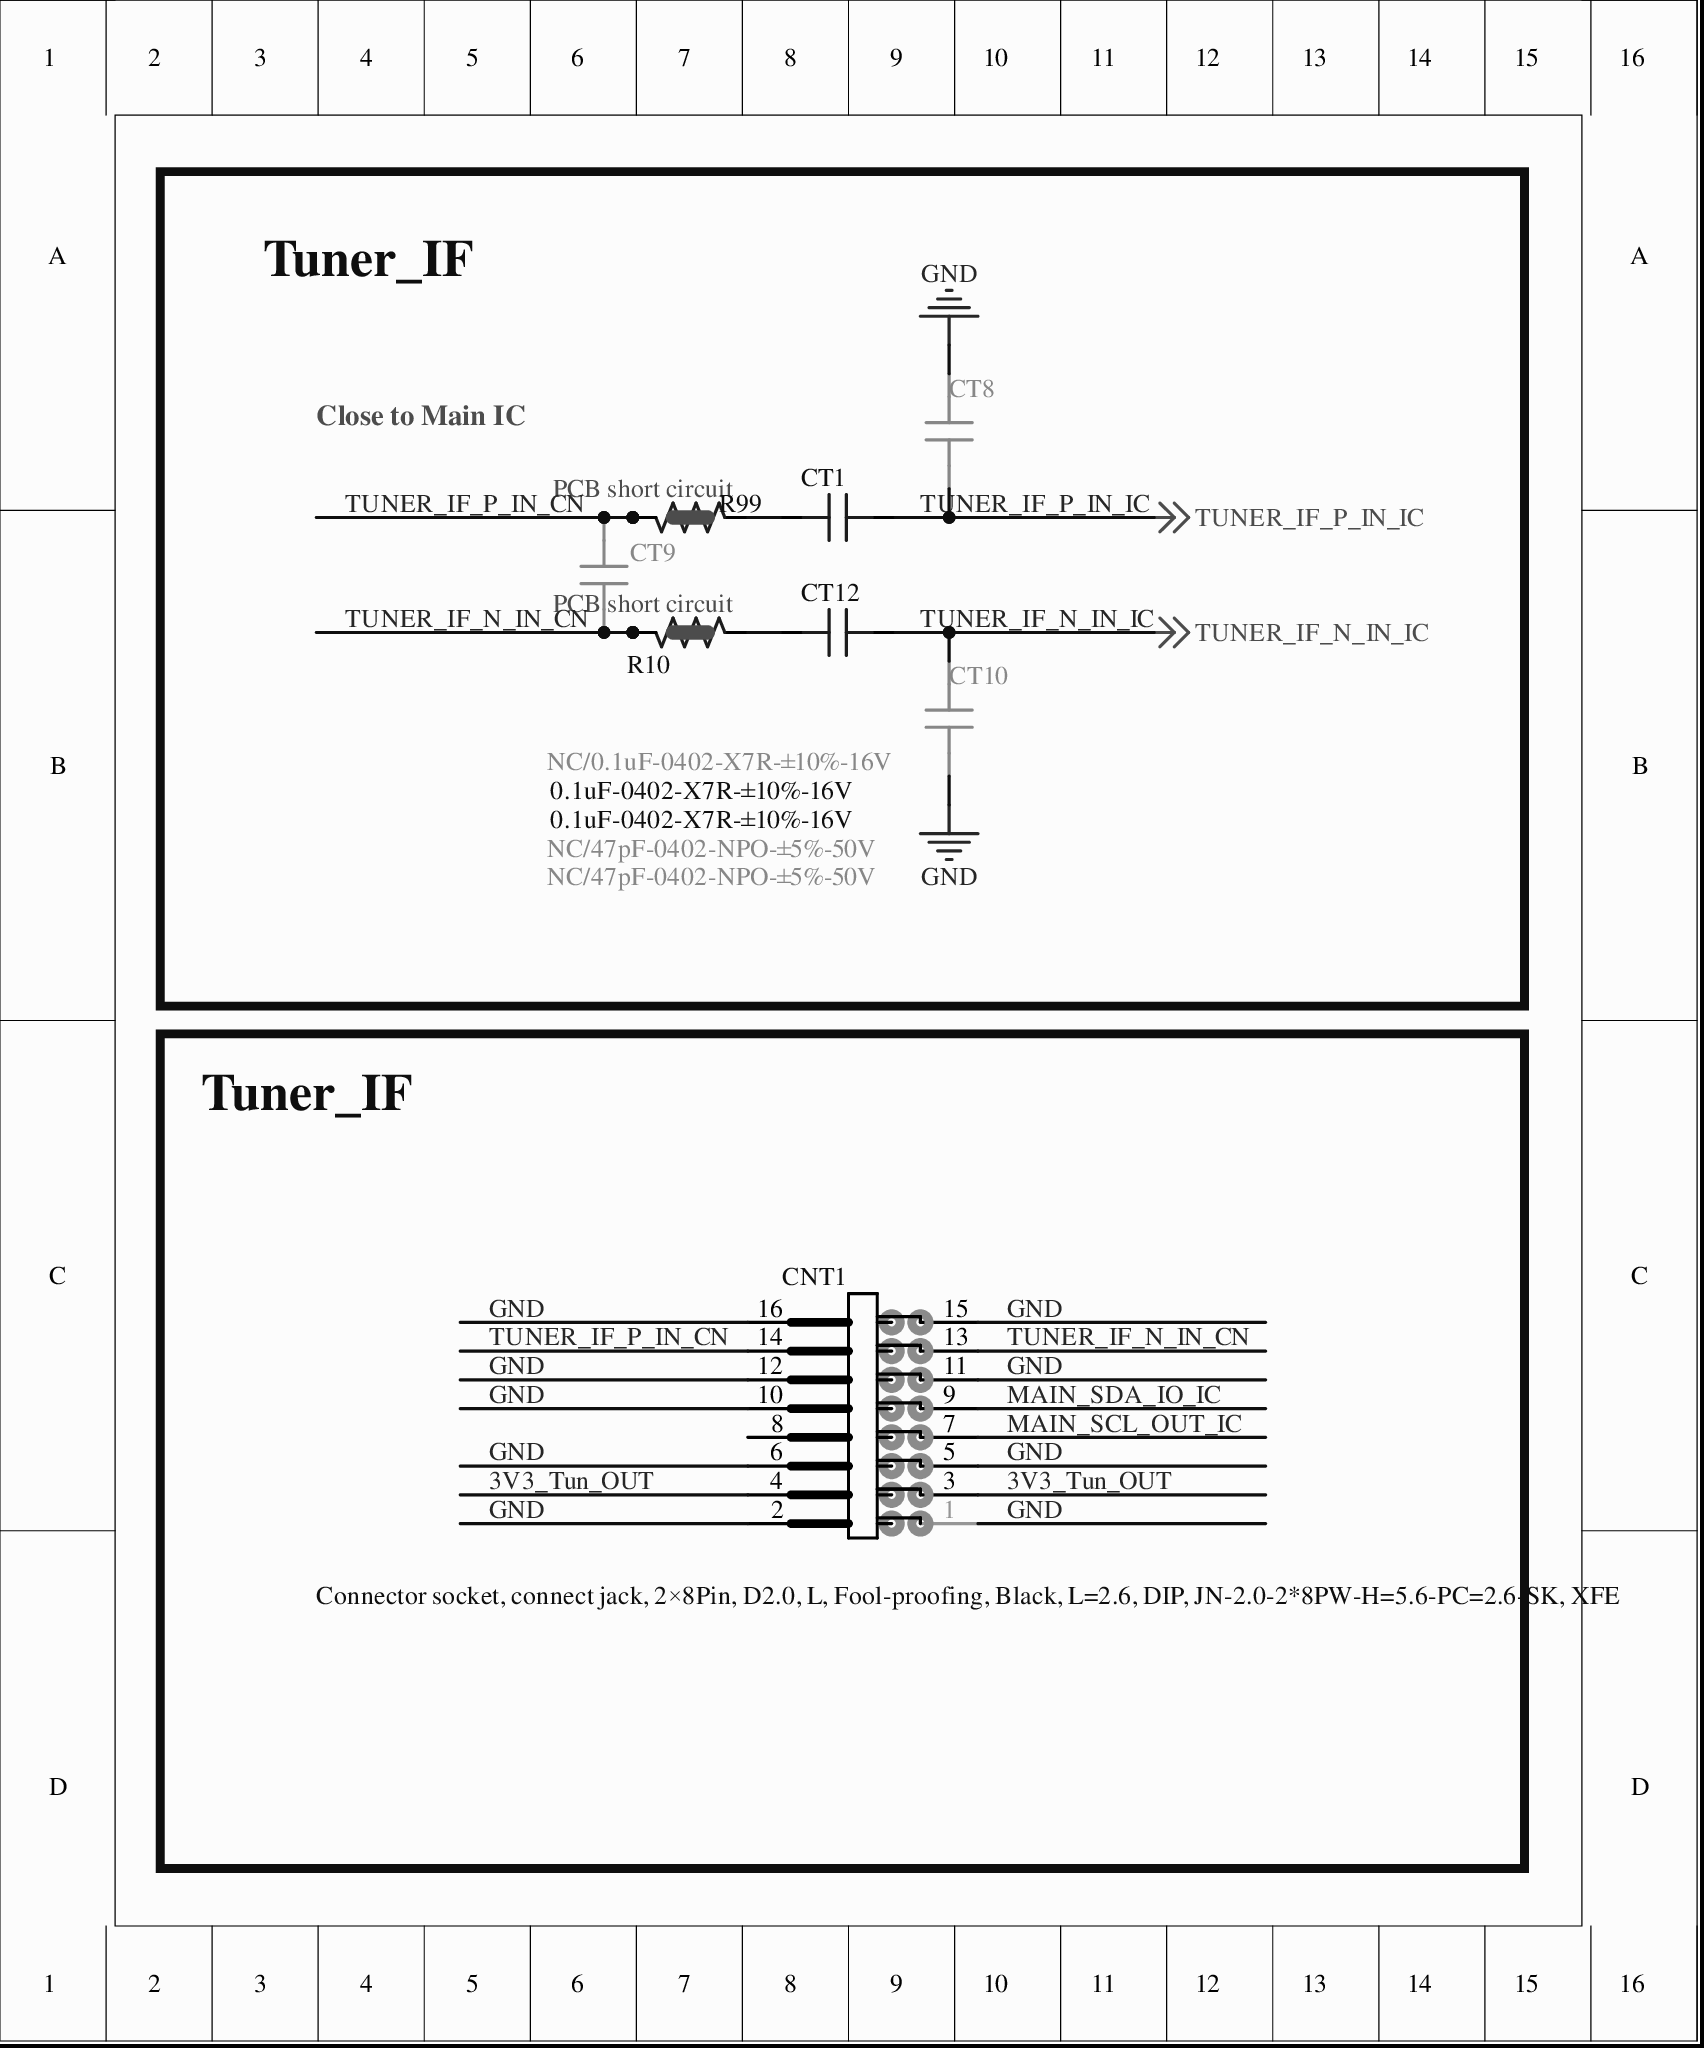
[diagram p0: MISC105950-42.SchDoc]
# Altium project MISC105950-48.PrjPCB (part 8 of 8)

## Sheet MISC105950-42.SchDoc
size 149 x 180 mm

### Parts
CNT1  Connector socket, connect jack, 2×8Pin, D2.0, L, Fool-proofing, Black, L=2.6, DIP, JN-2.0-2*8PW-H=5.6-PC=2.6-SK, XFE  [SIP2*8H/2.0DM-1]
CT1  0.1uF-0402-X7R-±10%-16V  [C0402]
CT8  NC/47pF-0402-NPO-±5%-50V  [C0402]
CT9  NC/0.1uF-0402-X7R-±10%-16V  [C0402]
CT10  NC/47pF-0402-NPO-±5%-50V  [C0402]
CT12  0.1uF-0402-X7R-±10%-16V  [C0402]
R10  NC/0ohm-0402-PCB  [R0402SC]  (value not drawn)
R99  NC/0ohm-0402-PCB  [R0402SC]  (value not drawn)

### Blocks framed on the sheet
Tuner_IF: CT1 CT8-CT10 CT12 R10 R99
Tuner_IF: CNT1

### Nets
3V3_Tun_OUT: CNT1.3 CNT1.4
GND: CNT1.1 CNT1.2 CNT1.5 CNT1.6 CNT1.10 CNT1.11 CNT1.12 CNT1.15 CNT1.16 CT8.1 CT10.2
MAIN_SCL_OUT_IC: CNT1.7
MAIN_SDA_IO_IC: CNT1.9
TUNER_IF_N_IN_CN: CNT1.13 CT9.1 R10.2 R10.3
TUNER_IF_N_IN_IC: CT10.1 CT12.1 ; off-sheet TUNER_IF_N_IN_IC
TUNER_IF_P_IN_CN: CNT1.14 CT9.2 R99.2 R99.3
TUNER_IF_P_IN_IC: CT1.1 CT8.2 ; off-sheet TUNER_IF_P_IN_IC
NetCT1_2: CT1.2 R99.1
NetCT12_2: CT12.2 R10.1

Not connected (* = marked no-connect by the designer): CNT1 8*

### Notes on the sheet
- Close to Main IC

### Library data of the parts
CNT1 = 连接插座-公座,male connect jack,2×8Pin,D2.0,L,Fool-proofing,Black,L=3.0mm,DIP,LK-DLMI
CT1 CT9 CT12 = 004.003.0000403-D: Ceramic capacitor, CAP MC, 16V, 0.1uF, ±20%, X5R, 0402, SMD, TP-D
CT8 CT10 = 004.003.0000556-D: Ceramic capacitor, CAP MC, 50V, 47pF, ±5%, NPO, 0402, SMD, TP-D
R10 R99 = 0ohm-0402-PCB-D

## Sheet MISC105950-43.SchDoc
size 416 x 279 mm
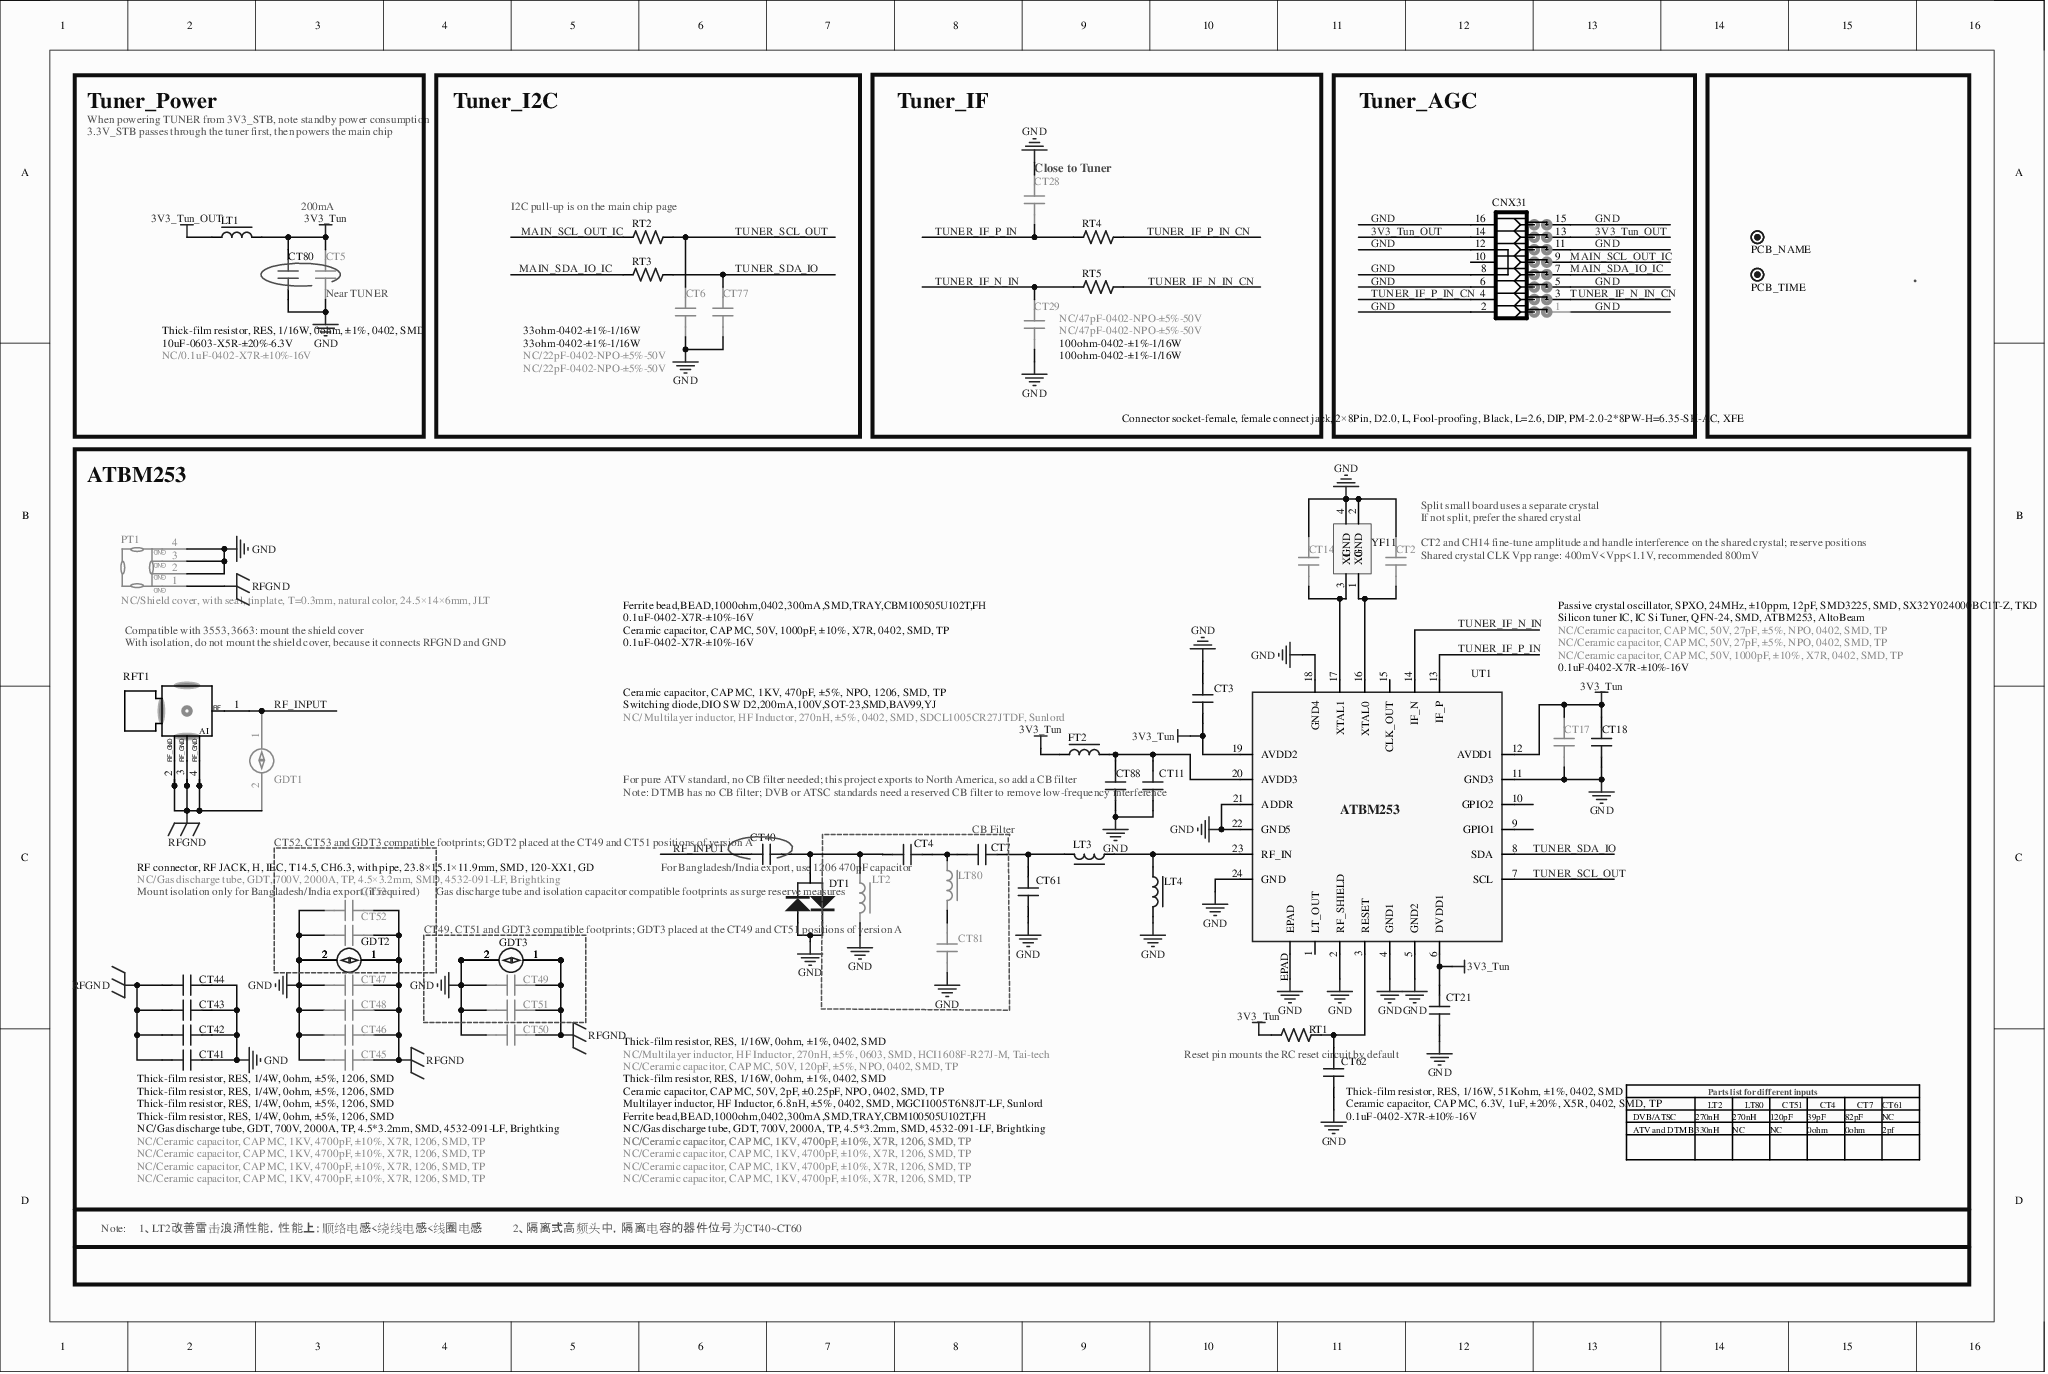
[diagram p1: MISC105950-43.SchDoc]

### Parts
CNX31  Connector socket-female, female connect jack, 2×8Pin, D2.0, L, Fool-proofing, Black, L=2.6, DIP, PM-2.0-2*8PW-H=6.35-SK-AC, XFE  [SIP2*8H/2.0DF-1]
CT2  NC/Ceramic capacitor, CAP MC, 50V, 27pF, ±5%, NPO, 0402, SMD, TP  [C0402]
CT3  0.1uF-0402-X7R-±10%-16V  [C0402]
CT4  Thick-film resistor, RES, 1/16W, 0ohm, ±1%, 0402, SMD  [C0402]
CT5  NC/0.1uF-0402-X7R-±10%-16V  [C0402]
CT6  NC/22pF-0402-NPO-±5%-50V  [C0402]
CT7  Thick-film resistor, RES, 1/16W, 0ohm, ±1%, 0402, SMD  [C0402]
CT11  Ceramic capacitor, CAP MC, 50V, 1000pF, ±10%, X7R, 0402, SMD, TP  [C0402]
CT14  NC/Ceramic capacitor, CAP MC, 50V, 27pF, ±5%, NPO, 0402, SMD, TP  [C0402]
CT17  NC/Ceramic capacitor, CAP MC, 50V, 1000pF, ±10%, X7R, 0402, SMD, TP  [C0402]
CT18  0.1uF-0402-X7R-±10%-16V  [C0402]
CT21  0.1uF-0402-X7R-±10%-16V  [C0402]
CT28  NC/47pF-0402-NPO-±5%-50V  [C0402]
CT29  NC/47pF-0402-NPO-±5%-50V  [C0402]
CT40  Ceramic capacitor, CAP MC, 1KV, 470pF, ±5%, NPO, 1206, SMD, TP  [C1206]
CT41  Thick-film resistor, RES, 1/4W, 0ohm, ±5%, 1206, SMD  [C1206]
CT42  Thick-film resistor, RES, 1/4W, 0ohm, ±5%, 1206, SMD  [C1206]
CT43  Thick-film resistor, RES, 1/4W, 0ohm, ±5%, 1206, SMD  [C1206]
CT44  Thick-film resistor, RES, 1/4W, 0ohm, ±5%, 1206, SMD  [C1206]
CT45  NC/Ceramic capacitor, CAP MC, 1KV, 4700pF, ±10%, X7R, 1206, SMD, TP  [C1206]
CT46  NC/Ceramic capacitor, CAP MC, 1KV, 4700pF, ±10%, X7R, 1206, SMD, TP  [C1206]
CT47  NC/Ceramic capacitor, CAP MC, 1KV, 4700pF, ±10%, X7R, 1206, SMD, TP  [C1206]
CT48  NC/Ceramic capacitor, CAP MC, 1KV, 4700pF, ±10%, X7R, 1206, SMD, TP  [C1206]
CT49  NC/Ceramic capacitor, CAP MC, 1KV, 4700pF, ±10%, X7R, 1206, SMD, TP  [C1206]
CT50  NC/Ceramic capacitor, CAP MC, 1KV, 4700pF, ±10%, X7R, 1206, SMD, TP  [C1206]
CT51  NC/Ceramic capacitor, CAP MC, 1KV, 4700pF, ±10%, X7R, 1206, SMD, TP  [C1206]
CT52  NC/Ceramic capacitor, CAP MC, 1KV, 4700pF, ±10%, X7R, 1206, SMD, TP  [C1206]
CT53  NC/Ceramic capacitor, CAP MC, 1KV, 4700pF, ±10%, X7R, 1206, SMD, TP  [C1206]
CT61  Ceramic capacitor, CAP MC, 50V, 2pF, ±0.25pF, NPO, 0402, SMD, TP  [C0402]
CT62  Ceramic capacitor, CAP MC, 6.3V, 1uF, ±20%, X5R, 0402, SMD, TP  [C0402]
CT77  NC/22pF-0402-NPO-±5%-50V  [C0402]
CT80  10uF-0603-X5R-±20%-6.3V  [C0603]
CT81  NC/Ceramic capacitor, CAP MC, 50V, 120pF, ±5%, NPO, 0402, SMD, TP  [C0402]
CT88  0.1uF-0402-X7R-±10%-16V  [C0402]
DT1  Switching diode,DIO SW D2,200mA,100V,SOT-23,SMD,BAV99,YJ  [SO-23]
FT2  Ferrite bead,BEAD,1000ohm,0402,300mA,SMD,TRAY,CBM100505U102T,FH  [L0402]
GDT1  NC/Gas discharge tube, GDT, 700V, 2000A, TP, 4.5×3.2mm, SMD, 4532-091-LF, Brightking  [SMD4532-1]
GDT2  NC/Gas discharge tube, GDT, 700V, 2000A, TP, 4.5*3.2mm, SMD, 4532-091-LF, Brightking  [SMD4532-1-C1206]
GDT3  NC/Gas discharge tube, GDT, 700V, 2000A, TP, 4.5*3.2mm, SMD, 4532-091-LF, Brightking  [SMD4532-1-C1206]
LT1  Thick-film resistor, RES, 1/16W, 0ohm, ±1%, 0402, SMD  [L0402]
LT2  NC/ Multilayer inductor, HF Inductor, 270nH, ±5%, 0402, SMD, SDCL1005CR27JTDF, Sunlord  [L0402]
LT3  Multilayer inductor, HF Inductor, 6.8nH, ±5%, 0402, SMD, MGCI1005T6N8JT-LF, Sunlord  [L0402]
LT4  Ferrite bead,BEAD,1000ohm,0402,300mA,SMD,TRAY,CBM100505U102T,FH  [L0402]
LT80  NC/Multilayer inductor, HF Inductor, 270nH, ±5%, 0603, SMD, HCI1608F-R27J-M, Tai-tech  [L0603]
PT1  NC/Shield cover, with seal, tinplate, T=0.3mm, natural color, 24.5×14×6mm, JLT  [SHIELD(24.5*14*6)-TEMP-NG]
RFT1  RF connector, RF JACK, H, IEC, T14.5, CH6.3, with pipe, 23.8×15.1×11.9mm, SMD, 120-XX1, GD  [T-12.8×10×9.3-IEC14.5-6.3]
RT1  Thick-film resistor, RES, 1/16W, 51Kohm, ±1%, 0402, SMD  [R0402]
RT2  33ohm-0402-±1%-1/16W  [R0402]
RT3  33ohm-0402-±1%-1/16W  [R0402]
RT4  100ohm-0402-±1%-1/16W  [R0402]
RT5  100ohm-0402-±1%-1/16W  [R0402]
UT1  Silicon tuner IC, IC Si Tuner, QFN-24, SMD, ATBM253, AltoBeam  [QFN24/0.4-1]
XX.XXXX  PCB_NAME  [PCB_NAME]
XXXXXX.  PCB_TIME  [PCB_TIME]
YF11  Passive crystal oscillator, SPXO, 24MHz, ±10ppm, 12pF, SMD3225, SMD, SX32Y024000BC1T-Z, TKD  [XTAL-S-3]

### Blocks framed on the sheet
Tuner_Power: CT5 CT80 LT1
Tuner_I2C: CT6 CT77 RT2 RT3
Tuner_IF: CT28 CT29 RT4 RT5
Tuner_AGC: CNX31
ATBM253: CT2 CT3 CT11 CT14 CT17 CT18 CT21 CT40-CT53 CT61 CT62 CT88 DT1 FT2 GDT1-GDT3 LT3 LT4 PT1 RFT1 RT1 UT1 YF11
CB Filter: CT4 CT7 CT81 LT2 LT80

### Nets
3V3_Tun: CT3.2 CT5.1 CT17.1 CT18.2 CT21.2 CT80.2 FT2.2 LT1.2 RT1.1 UT1.6(DVDD1) UT1.12(AVDD1) UT1.19(AVDD2)
3V3_Tun_OUT: CNX31.13 CNX31.14 LT1.1
GND: CNX31.1 CNX31.2 CNX31.5 CNX31.6 CNX31.8 CNX31.11 CNX31.12 CNX31.15 CNX31.16 CT2.1 CT3.1 CT5.2 CT6.1 CT11.1 CT14.1 CT17.2 CT18.1 CT21.1 CT28.1 CT29.2 CT41.1 CT42.1 CT43.1 CT44.1 CT45.2 CT46.2 CT47.2 CT48.2 CT49.2 CT50.2 CT51.2 CT52.2 CT53.2 CT61.2 CT62.2 CT77.1 CT80.1 CT81.2 CT88.2 DT1.1 DT1.3 GDT2.2 GDT3.2 LT2.1 LT4.1 PT1.2 PT1.3 PT1.4 UT1.2(RF_SHIELD) UT1.4(GND1) UT1.5(GND2) UT1.11(GND3) UT1.18(GND4) UT1.21(ADDR) UT1.22(GND5) UT1.24(GND) UT1.EPAD YF11.2(GND) YF11.4(GND)
RFGND: CT41.2 CT42.2 CT43.2 CT44.2 CT45.1 CT46.1 CT47.1 CT48.1 CT49.1 CT50.1 CT51.1 CT52.1 CT53.1 GDT1.2 GDT2.1 GDT3.1 PT1.1 RFT1.2 RFT1.3 RFT1.4
MAIN_SCL_OUT_IC: CNX31.9 RT2.1
MAIN_SDA_IO_IC: CNX31.7 RT3.1
RF_INPUT: CT40.1 GDT1.1 RFT1.1
TUNER_IF_N_IN: CT29.1 RT5.1 UT1.14(IF_N)
TUNER_IF_N_IN_CN: CNX31.3 RT5.2
TUNER_IF_P_IN: CT28.2 RT4.1 UT1.13(IF_P)
TUNER_IF_P_IN_CN: CNX31.4 RT4.2
TUNER_SCL_OUT: CT6.2 RT2.2 UT1.7(SCL)
TUNER_SDA_IO: CT77.2 RT3.2 UT1.8(SDA)
NetCT2_2: CT2.2 UT1.16(XTAL0) YF11.1(X0)
NetCT4_1: CT4.1 CT7.2 LT80.1
NetCT4_2: CT4.2 CT40.2 DT1.2 LT2.2
NetCT7_1: CT7.1 CT61.1 LT3.1
NetCT11_2: CT11.2 CT88.1 FT2.1 UT1.20(AVDD3)
NetCT14_2: CT14.2 UT1.17(XTAL1) YF11.3(XI)
NetCT62_1: CT62.1 RT1.2 UT1.3(RESET)
NetCT81_1: CT81.1 LT80.2
NetLT3_2: LT3.2 LT4.2 UT1.23(RF_IN)

Not connected (* = marked no-connect by the designer): CNX31 10*; UT1 1(LT_OUT)* 9(GPIO1)* 10(GPIO2)* 15(CLK_OUT)*

### Notes on the sheet
- When powering TUNER from 3V3_STB, note standby power consumption
- 3.3V_STB passes through the tuner first, then powers the main chip
- 200mA
- (near RT2) I2C pull-up is on the main chip page
- (near CT28) Close to Tuner
- (near CT5) Near TUNER
- Split small board uses a separate crystal
- (near CT2) If not split, prefer the shared crystal
- (near CT2) CT2 and CH14 fine-tune amplitude and handle interference on the shared crystal; reserve positions
- (near CT2) Shared crystal CLK Vpp range: 400mV<Vpp<1.1V, recommended 800mV
- (near PT1) Compatible with 3553, 3663: mount the shield cover
- With isolation, do not mount the shield cover, because it connects RFGND and GND
- For pure ATV standard, no CB filter needed; this project exports to North America, so add a CB filter
- Note: DTMB has no CB filter; DVB or ATSC standards need a reserved CB filter to remove low-frequency interference
- (near CT53) Mount isolation only for Bangladesh/India export (if required)
- (near CT40) CT52, CT53 and GDT3 compatible footprints; GDT2 placed at the CT49 and CT51 positions of version A
- Gas discharge tube and isolation capacitor compatible footprints as surge reserve measures
- (near LT80) For Bangladesh/India export, use 1206 470pF capacitor
- (near CT81) CT49, CT51 and GDT3 compatible footprints; GDT3 placed at the CT49 and CT51 positions of version A
- (near CT62) Reset pin mounts the RC reset circuit by default
- DVB/ATSC
- ATV and DTMB
- 270nH
- 330nH
- LT2
- Parts list for different inputs
- NC
- LT80
- 120pF
- CT51
- 39pF
- 0ohm
- CT4
- 82pF
- CT7
- CT61
- 2pf
- Note:
- 1、LT2改善雷击浪涌性能，性能上：顺络电感<绕线电感<线圈电感
- 2、隔离式高频头中，隔离电容的器件位号为CT40~CT60

### Library data of the parts
CNX31 = 连接插座-母座,female connect jack,2×8Pin,D2.0,L,Fool-proofing,Black,L=2.6mm,DIP,LK-DLMI
CT2-CT4 CT7 CT11 CT14 CT17 CT18 CT21 CT61 CT62 CT81 CT88 = 0.1uF-0402-Y5V-+80%-20%-16V-D
CT5 = 1uF-0402-X5R-±20%-6.3V-D
CT6 CT77 = 004.003.0000530-D: Ceramic capacitor, CAP MC, 50V, 22pF, ±5%, NPO, 0402, SMD, TP-D
CT28 CT29 = 004.003.0000556-D: as CT8 on sheet MISC105950-42
CT40 = 0.47uF-1206-Y5V-+80%-20%-16V-D
CT41-CT53 = 1000pF-1206-X7R-±20%-2000V-D
CT80 = 004.003.0000383-D: Ceramic capacitor, CAP MC, 6.3V, 10uF, ±20%, X5R, 0603, SMD, TP-D
DT1 = BAV99-BR-D
FT2 LT2-LT4 = SDCL1005CR27JTDF(顺络)-D
GDT1 = 004.005.0000675: Gas discharge tube, GDT, 700V, 2000A, TP, 4.5*3.2mm, SMD, 4532-091-LF, Brightking-D
GDT2 GDT3 = 004.005.0000675-C1206: Gas discharge tube, GDT, 700V, 2000A, TP, 4.5*3.2mm, SMD, 4532-091-LF, Brightking-D
LT1 = 004.004.0000335-D: Ferrite bead,BEAD,120ohm,0402,500mA,SMD,TP,GZ1005U121CTF,Sunlord-D
LT80 = MGLB1608M121T2R0-LF(120ohm-2000mA)-D
PT1 = 004.040.0007718-DLMI: MB shield cover 2, D716AF, 48.9×33.9×3.3mm, SPET, natural color, QX-DLMI
RFT1 = XXX.XXX.0005128-D: RF connector, RF JACK, H, IEC, T14.5, CH6.3, with pipe, 23.8×15.1×11.9mm, SMD, 120-XX1, GD-D
RT1-RT5 = 004.002.0000568-D: Thick-film resistor, RES, 1/16W, 100ohm, ±5%, 0402, SMD-D
UT1 = 004.014.0000255-D: Silicon tuner IC, IC Si Tuner, QFN-24, SMD, ATBM253, AltoBeam-D
YF11 = 16.000MHz±20PPM-10PF-SMD3225-D: NC: GPS; PCB DECAL: TCXO_3225; Source_Path: EM_66_V2.0_201209181010.DSN; Value: 26M/0.5PPM/1.8V

## Nets that join several sheets
3V3_STB: MISC105950-35 (7 pins), MISC105950-36 (27 pins), MISC105950-37 (RK1.1 RK2.2 RK13.2 RK25.2), MISC105950-38 (RF4.2), MISC105950-40 (RH101.2 RH104.2 RH106.2), MISC105950-44 (RA51.2 RA61.1)
3V3_Tun_OUT: MISC105950-35 (5 pins), MISC105950-42 (CNT1.3 CNT1.4), MISC105950-43 (CNX31.13 CNX31.14 LT1.1)
5V_M: MISC105950-35 (10 pins), MISC105950-39 (FU1.2 RO31.2 RU1.2), MISC105950-44 (RA70.2)
5V_STB: MISC105950-35 (19 pins), MISC105950-37 (RK10.2)
12V/15V: MISC105950-35 (19 pins), MISC105950-38 (CW7.2 QW3.S RW10.2), MISC105950-41 (12 pins)
+1.8V_DDR: MISC105950-35 (5 pins), MISC105950-36 (8 pins)
GND: MISC105950-31 (24 pins), MISC105950-35 (68 pins), MISC105950-36 (41 pins), MISC105950-37 (15 pins), MISC105950-38 (21 pins), MISC105950-39 (50 pins), MISC105950-40 (66 pins), MISC105950-41 (31 pins), MISC105950-44 (22 pins), MISC105950-42 (11 pins), MISC105950-43 (59 pins)
VCC_PANEL: MISC105950-35 (6 pins), MISC105950-38 (10 pins)
VDDC_CORE: MISC105950-35 (7 pins), MISC105950-36 (14 pins)
ADIM_OUT_IC: MISC105950-35 (CG5.2 RG1.2 RG29.1), MISC105950-36 (U1.90)
AMP_L_OUT_IC: MISC105950-36 (CF29.1 U1.41), MISC105950-44 (CA29.1 CA59.1 CA64.1)
AMP_MUTE_OUT_IC: MISC105950-36 (U1.56), MISC105950-41 (RA1.1 RA2.2)
AMP_R_OUT_IC: MISC105950-36 (CF30.1 U1.42), MISC105950-44 (CA31.1 CA60.1 CA63.1)
AV1_CVBS_IN_IC: MISC105950-36 (U1.31), MISC105950-39 (CI33.2)
AV_L_IN_IC: MISC105950-36 (U1.37), MISC105950-39 (CI3.1)
AV_R_IN_IC: MISC105950-36 (U1.38), MISC105950-39 (CI4.1)
BRI_ADJ: MISC105950-35 (CG6.2 RG2.2), MISC105950-36 (RF29.1 U1.95)
EPH_SDN_OUT_IC: MISC105950-36 (U1.53), MISC105950-44 (RA68.1)
HDMI_A_0N_IN_IC: MISC105950-36 (U1.1), MISC105950-40 (JH23.9 UH70.3 UH70.6)
HDMI_A_0P_IN_IC: MISC105950-36 (U1.2), MISC105950-40 (JH23.7 UH70.4 UH70.5)
HDMI_A_1N_IN_IC: MISC105950-36 (U1.3), MISC105950-40 (JH23.6 UH71.1 UH71.8)
HDMI_A_1P_IN_IC: MISC105950-36 (U1.4), MISC105950-40 (JH23.4 UH71.2 UH71.7)
HDMI_A_2N_IN_IC: MISC105950-36 (U1.5), MISC105950-40 (JH23.3 UH71.3 UH71.6)
HDMI_A_2P_IN_IC: MISC105950-36 (U1.6), MISC105950-40 (JH23.1 UH71.4 UH71.5)
HDMI_A_CKN_IN_IC: MISC105950-36 (U1.127), MISC105950-40 (JH23.12 UH70.1 UH70.8)
HDMI_A_CKP_IN_IC: MISC105950-36 (U1.128), MISC105950-40 (JH23.10 UH70.2 UH70.7)
HDMI_A_HPD_OUT_IC: MISC105950-36 (U1.120), MISC105950-40 (RH71.5 RH71.7)
HDMI_A_SCL_IN_IC: MISC105950-36 (U1.107), MISC105950-40 (RH72.2)
HDMI_A_SDA_IO_IC: MISC105950-36 (U1.106), MISC105950-40 (RH73.2)
HDMI_ARC_OUT_IC: MISC105950-36 (U1.125), MISC105950-40 (CH81.2)
HDMI_B_0N_IN_IC: MISC105950-36 (U1.9), MISC105950-40 (JH22.9 UH21.3 UH21.6)
HDMI_B_0P_IN_IC: MISC105950-36 (U1.10), MISC105950-40 (JH22.7 UH21.4 UH21.5)
HDMI_B_1N_IN_IC: MISC105950-36 (U1.11), MISC105950-40 (JH22.6 UH22.1 UH22.8)
HDMI_B_1P_IN_IC: MISC105950-36 (U1.12), MISC105950-40 (JH22.4 UH22.2 UH22.7)
HDMI_B_2N_IN_IC: MISC105950-36 (U1.13), MISC105950-40 (JH22.3 UH22.3 UH22.6)
HDMI_B_2P_IN_IC: MISC105950-36 (U1.14), MISC105950-40 (JH22.1 UH22.4 UH22.5)
HDMI_B_CKN_IN_IC: MISC105950-36 (U1.7), MISC105950-40 (JH22.12 UH21.1 UH21.8)
HDMI_B_CKP_IN_IC: MISC105950-36 (U1.8), MISC105950-40 (JH22.10 UH21.2 UH21.7)
HDMI_B_HPD_OUT_IC: MISC105950-36 (U1.121), MISC105950-40 (RH24.5 RH24.7)
HDMI_B_SCL_IN_IC: MISC105950-36 (U1.116), MISC105950-40 (RH35.4)
HDMI_B_SDA_IO_IC: MISC105950-36 (U1.115), MISC105950-40 (RH35.2)
HDMI_C_0N_IN_IC: MISC105950-36 (U1.18), MISC105950-40 (JH21.9 UH1.3 UH1.6)
HDMI_C_0P_IN_IC: MISC105950-36 (U1.19), MISC105950-40 (JH21.7 UH1.4 UH1.5)
HDMI_C_1N_IN_IC: MISC105950-36 (U1.20), MISC105950-40 (JH21.6 UH2.1 UH2.8)
HDMI_C_1P_IN_IC: MISC105950-36 (U1.21), MISC105950-40 (JH21.4 UH2.2 UH2.7)
HDMI_C_2N_IN_IC: MISC105950-36 (U1.22), MISC105950-40 (JH21.3 UH2.3 UH2.6)
HDMI_C_2P_IN_IC: MISC105950-36 (U1.23), MISC105950-40 (JH21.1 UH2.4 UH2.5)
HDMI_C_CKN_IN_IC: MISC105950-36 (U1.16), MISC105950-40 (JH21.12 UH1.1 UH1.8)
HDMI_C_CKP_IN_IC: MISC105950-36 (U1.17), MISC105950-40 (JH21.10 UH1.2 UH1.7)
HDMI_C_HPD_OUT_IC: MISC105950-36 (U1.122), MISC105950-40 (RH34.2 RH34.4)
HDMI_C_SCL_IN_IC: MISC105950-36 (U1.118), MISC105950-40 (RH35.8)
HDMI_C_SDA_IO_IC: MISC105950-36 (U1.117), MISC105950-40 (RH35.6)
HDMI_CEC_IO_IC: MISC105950-36 (U1.119), MISC105950-40 (DH4.K RH83.1)
HDMIA_DET_IC: MISC105950-36 (U1.110), MISC105950-40 (CH72.2 RH74.1 RH75.1)
HDMIB_DET_IC: MISC105950-36 (U1.91), MISC105950-40 (CH60.2 RH1.1 RH2.1)
HDMIC_DET_IC: MISC105950-36 (U1.92), MISC105950-40 (CH3.2 RH81.1 RH82.1)
HP_DET_IC: MISC105950-36 (U1.58), MISC105950-44 (CA99.2 RA52.2)
IR_IN_IC: MISC105950-36 (U1.97), MISC105950-37 (CK1.2 RK6.2)
KEY_IN_IC: MISC105950-36 (U1.109), MISC105950-37 (CK11.1 RK23.1)
LED_R_OUT_IC: MISC105950-36 (U1.59), MISC105950-37 (RK13.1 RK14.1 RK15.1)
LINE_L_OUT_IC: MISC105950-36 (U1.39), MISC105950-41 (RA3.1)
LINE_R_OUT_IC: MISC105950-36 (U1.40), MISC105950-41 (RA14.1)
LVDS_E0N_IC: MISC105950-36 (U1.76), MISC105950-38 (CN22.24 E0N.1)
LVDS_E0P_IC: MISC105950-36 (U1.75), MISC105950-38 (CN22.23 E0P.1)
LVDS_E1N_IC: MISC105950-36 (U1.74), MISC105950-38 (CN22.22 E1N.1)
LVDS_E1P_IC: MISC105950-36 (U1.73), MISC105950-38 (CN22.21 E1P.1)
LVDS_E2N_IC: MISC105950-36 (U1.72), MISC105950-38 (CN22.20 E2N.1)
LVDS_E2P_IC: MISC105950-36 (U1.71), MISC105950-38 (CN22.19 E2P.1)
LVDS_E3N_IC: MISC105950-36 (U1.68), MISC105950-38 (CN22.14 E3N.1)
LVDS_E3P_IC: MISC105950-36 (U1.67), MISC105950-38 (CN22.13 E3P.1)
LVDS_E4N_IC: MISC105950-36 (U1.66), MISC105950-38 (CN22.12 E4N.1)
LVDS_E4P_IC: MISC105950-36 (U1.65), MISC105950-38 (CN22.11 E4P.1)
LVDS_ECKN_IC: MISC105950-36 (U1.70), MISC105950-38 (CF94.2 CN22.17 ECKN.1)
LVDS_ECKP_IC: MISC105950-36 (U1.69), MISC105950-38 (CF71.2 CN22.16 ECKP.1)
LVDS_O0N_IC: MISC105950-36 (U1.89), MISC105950-38 (CN22.40 O0N.1)
LVDS_O0P_IC: MISC105950-36 (U1.88), MISC105950-38 (CN22.39 O0P.1)
LVDS_O1N_IC: MISC105950-36 (U1.87), MISC105950-38 (CN22.38 O1N.1)
LVDS_O1P_IC: MISC105950-36 (U1.86), MISC105950-38 (CN22.37 O1P.1)
LVDS_O2N_IC: MISC105950-36 (U1.84), MISC105950-38 (CN22.36 O2N.1)
LVDS_O2P_IC: MISC105950-36 (U1.83), MISC105950-38 (CN22.35 O2P.1)
LVDS_O3N_IC: MISC105950-36 (U1.80), MISC105950-38 (CN22.30 O3N.1)
LVDS_O3P_IC: MISC105950-36 (U1.79), MISC105950-38 (CN22.29 O3P.1)
LVDS_O4N_IC: MISC105950-36 (U1.78), MISC105950-38 (CN22.28 O4N.1)
LVDS_O4P_IC: MISC105950-36 (U1.77), MISC105950-38 (CN22.27 O4P.1)
LVDS_OCKN_IC: MISC105950-36 (U1.82), MISC105950-38 (CF96.2 CN22.33 OCKN.1)
LVDS_OCKP_IC: MISC105950-36 (U1.81), MISC105950-38 (CF95.2 CN22.32 OCKP.1)
MAIN_SCL_OUT_IC: MISC105950-36 (DK3.K RF43.2 U1.52), MISC105950-42 (CNT1.7), MISC105950-43 (CNX31.9 RT2.1)
MAIN_SDA_IO_IC: MISC105950-36 (DK2.K RF44.2 U1.51), MISC105950-42 (CNT1.9), MISC105950-43 (CNX31.7 RT3.1)
PANEL_EN_OUT_IC: MISC105950-35 (RD1.1 RD28.2), MISC105950-36 (U1.93), MISC105950-38 (RW13.1)
POWER_EN_OUT_IC: MISC105950-35 (RD46.1 RM1.1 RM2.1), MISC105950-36 (U1.57)
PWM1: MISC105950-35 (DI3.K RG3.2), MISC105950-36 (RF13.1 U1.96)
SPDIF_OUT_IC: MISC105950-36 (U1.94), MISC105950-39 (CO21.2 RO21.1)
TUNER_IF_N_IN_CN: MISC105950-42 (CNT1.13 CT9.1 R10.2 R10.3), MISC105950-43 (CNX31.3 RT5.2)
TUNER_IF_N_IN_IC: MISC105950-36 (U1.45), MISC105950-42 (CT10.1 CT12.1)
TUNER_IF_P_IN_CN: MISC105950-42 (CNT1.14 CT9.2 R99.2 R99.3), MISC105950-43 (CNX31.4 RT4.2)
TUNER_IF_P_IN_IC: MISC105950-36 (U1.44), MISC105950-42 (CT1.1 CT8.2)
UART_RX_IC: MISC105950-36 (U1.104), MISC105950-40 (CD101.K RH105.2 RH106.1)
UART_TX_IC: MISC105950-36 (U1.103), MISC105950-40 (CD102.K RH103.2 RH104.1)
USB0_DM_IO_IC: MISC105950-36 (U1.63), MISC105950-39 (DU31.K RU11.1)
USB0_DP_IO_IC: MISC105950-36 (U1.64), MISC105950-39 (DU32.K RU12.1)
USB1_DM_IO_IC: MISC105950-36 (U1.61), MISC105950-39 (DU33.K RU2.1)
USB1_DP_IO_IC: MISC105950-36 (U1.62), MISC105950-39 (DU34.K RU3.1)
YPBPR_PB_IN_IC: MISC105950-36 (U1.26), MISC105950-39 (CI95.2)
YPBPR_PR_IN_IC: MISC105950-36 (U1.29), MISC105950-39 (CI93.2)
YPBPR_Y_IN_IC: MISC105950-36 (U1.27), MISC105950-39 (CI98.2)